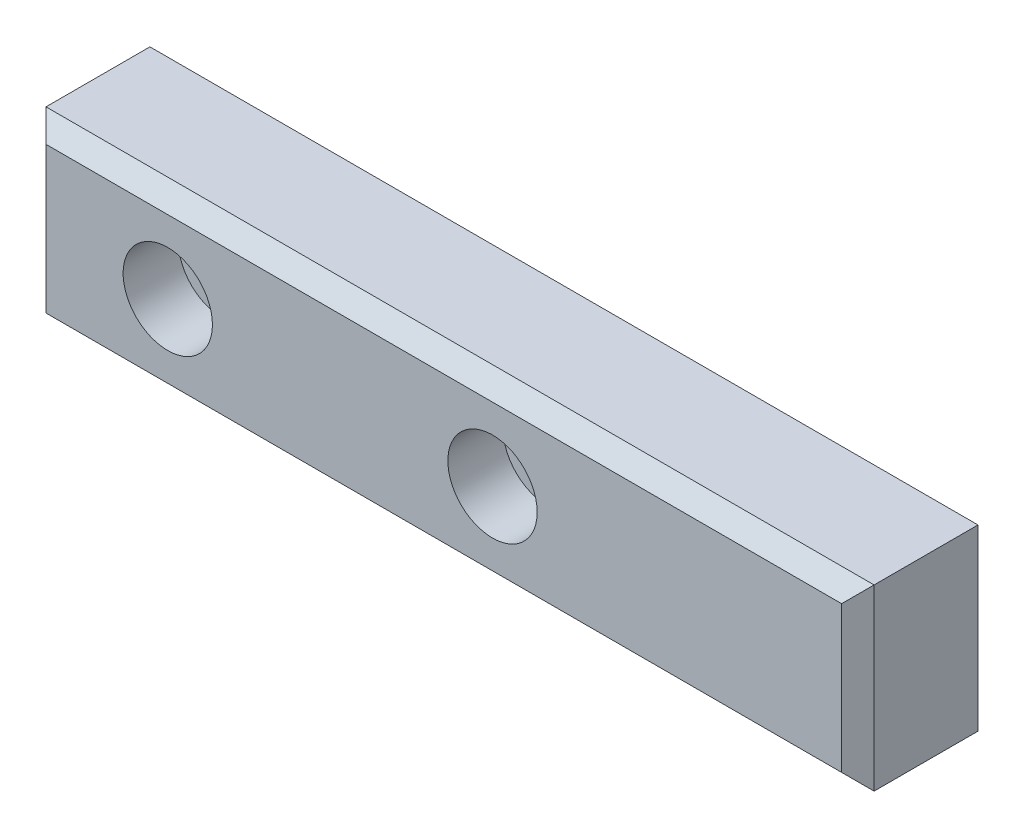
from build123d import *

# Parameters (mm, degrees)
SKETCH1_W                                            = 102
SKETCH1_H                                            = 22
BOSS_EXTRUDE1_DEPTH                                  = 15
HOLE_SIZE_PER_SOCKET_HEAD_CAP_SCREW_TYPE_D           = 6.6
HOLE_SIZE_PER_SOCKET_HEAD_CAP_SCREW_TYPE_CBORE_D     = 11
HOLE_SIZE_PER_SOCKET_HEAD_CAP_SCREW_TYPE_CBORE_DEPTH = 6.8
CHAMFER1_SIZE                                        = 0.2
CHAMFER2_SIZE                                        = 2


with BuildPart() as part:
    # Sketch1 → Boss-Extrude1 (new body)
    with BuildSketch(Plane.XY):
        Rectangle(SKETCH1_W, SKETCH1_H)
    extrude(amount=BOSS_EXTRUDE1_DEPTH)

    # Hole size per socket head cap screw type1 (through all)
    with Locations(Plane(origin=(-34, 0, 15), x_dir=(1, 0, 0), z_dir=(0, 0, 1))):
        with Locations((0, 0), (40, 0)):
            CounterBoreHole(HOLE_SIZE_PER_SOCKET_HEAD_CAP_SCREW_TYPE_D / 2, HOLE_SIZE_PER_SOCKET_HEAD_CAP_SCREW_TYPE_CBORE_D / 2, HOLE_SIZE_PER_SOCKET_HEAD_CAP_SCREW_TYPE_CBORE_DEPTH)

    # Chamfer1
    chamfer1_edges = [part.edges().sort_by_distance(p)[0] for p in [
        (0, 11, 0),
        (51, 0, 0),
        (0, -11, 0),
        (-51, 0, 0),
    ]]
    chamfer(chamfer1_edges, length=CHAMFER1_SIZE)

    # Chamfer2
    chamfer2_edges = [part.edges().sort_by_distance(p)[0] for p in [
        (51, 0, 15),
        (0, 11, 15),
        (-51, 0, 15),
        (0, -11, 15),
    ]]
    chamfer(chamfer2_edges, length=CHAMFER2_SIZE)


solid = part.part
